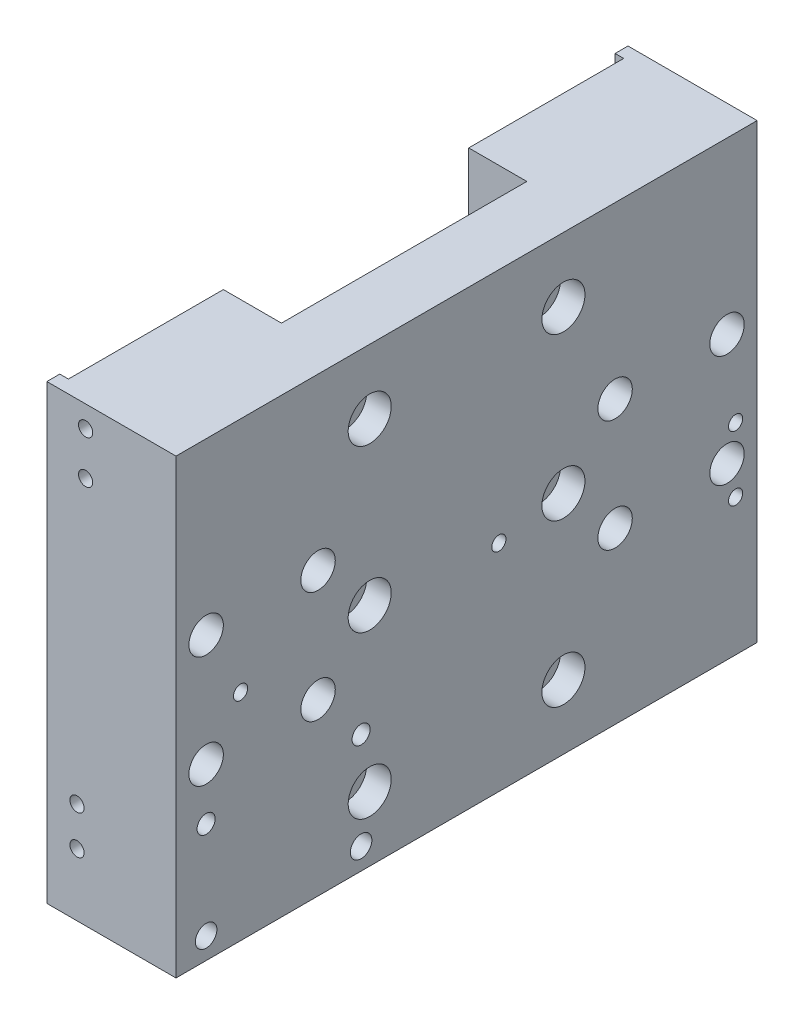
SolidWorks part; units mm, degrees
material "AL6061"
ref_plane "Front Plane" through (0, 0, 0) normal (0, 0, 1) x (1, 0, 0)
ref_plane "Top Plane" through (0, 0, 0) normal (0, 1, 0) x (1, 0, 0)
ref_plane "Right Plane" through (0, 0, 0) normal (1, 0, 0) x (0, 0, -1)
sketch "Sketch1" plane through (0, 0, 0) normal (1, 0, 0) x (0, 0, -1)
  line L1 (-67.5, -52.5) -> (67.5, -52.5)
  line L2 (-67.5, -52.5) -> (-67.5, 52.5)
  line L3 (-67.5, 52.5) -> (67.5, 52.5)
  line L4 (67.5, -52.5) -> (67.5, 52.5)
  line L5 (-67.5, -52.5) -> (67.5, 52.5) construction
  line L6 (-67.5, 52.5) -> (67.5, -52.5) construction
  point P0 (0, 0)
  dimension "D1" = 105
  dimension "D2" = 135
extrude "Boss-Extrude1" add sketch "Sketch1" along normal blind 30
sketch "Sketch2" plane through (0, -52.5, 0) normal (0, -1, 0) x (1, 0, 0)
  line L0 (0, 0) -> (30, 0) construction
  line L2 (0, 67.5) -> (0, -67.5) construction
  line L3 (15.5, -28.5) -> (0, -28.5)
  line L4 (15.5, -28.5) -> (15.5, 28.5)
  line L5 (15.5, 28.5) -> (0, 28.5)
  line L6 (0, -28.5) -> (0, 28.5)
  line L7 (15.5, -28.5) -> (0, 28.5) construction
  line L8 (15.5, 28.5) -> (0, -28.5) construction
  point P5 (7.75, 0)
  dimension "D1" = 57
  dimension "D2" = 15.5
extrude "Cut-Extrude1" cut sketch "Sketch2" against normal through all
sketch "Sketch3" plane through (0, 0, 0) normal (-1, 0, 0) x (0, 0, 1)
  line L0 (0, 52.5) -> (0, -52.5) construction
  line L3 (28.5, 52.5) -> (67.5, 52.5) construction
  line L4 (-64.5, -52.5) -> (64.5, -52.5)
  line L5 (-64.5, -52.5) -> (-64.5, 52.5)
  line L6 (-64.5, 52.5) -> (64.5, 52.5)
  line L7 (64.5, -52.5) -> (64.5, 52.5)
  line L8 (-64.5, -52.5) -> (64.5, 52.5) construction
  line L9 (-64.5, 52.5) -> (64.5, -52.5) construction
  point P6 (0, 0)
  dimension "D1" = 129
extrude "Cut-Extrude2" cut sketch "Sketch3" against normal blind 2
hole_wizard "CBORE for M5 Hexagon socket head cap screws1" positions "Sketch16" profile "Sketch17" counterbore size "M5" standard "GB" end condition through all
sketch "Sketch16" plane through (30, 0, 0) normal (1, 0, 0) x (0, 0, -1)
  line L0 (0, 52.5) -> (0, -52.5) construction
  line L1 (67.5, 52.5) -> (-67.5, 52.5) construction
  line L2 (-67.5, -52.5) -> (67.5, -52.5) construction
  line L3 (67.5, 0) -> (-67.5, 0) construction
  line L4 (67.5, -52.5) -> (67.5, 52.5) construction
  line L5 (-67.5, 52.5) -> (-67.5, -52.5) construction
  point P9 (22.5, 37.5)
  point P11 (-22.5, 37.5)
  point P23 (-22.5, 0)
  point P25 (22.5, 0)
  point P30 (-22.5, -37.5)
  point P31 (22.5, -37.5)
  dimension "D1" = 45
  dimension "D2" = 37.5
sketch "Sketch17" plane through (30, -37.5, -22.5) normal (0, 1, 0) x (0, 0, -1)
  line L0 (0, 0) -> (0, 30)
  line L1 (0, 30) -> (2.75, 30)
  line L3 (2.75, 30) -> (2.75, 5.7)
  line L4 (2.75, 5.7) -> (5, 5.7)
  line L5 (5, 5.7) -> (5, 0)
  line L7 (5, 0) -> (0, 0)
  line L11 (0, -6.35) -> (0, 107.95) construction
  dimension "通孔孔直径" = 5.5
  dimension "通孔孔深度" = 30
  dimension "柱形沉头孔直径" = 10
  dimension "柱形沉头孔深度" = 5.7
hole_wizard "CBORE for M4 Hexagon socket head cap screws1" positions "Sketch22" profile "Sketch23" counterbore size "M4" standard "GB" end condition through all
sketch "Sketch22" plane through (30, 0, 0) normal (1, 0, 0) x (0, 0, -1)
  line L0 (67.5, 0) -> (-67.5, 0) construction
  line L1 (67.5, -52.5) -> (67.5, 52.5) construction
  line L2 (-67.5, 52.5) -> (-67.5, -52.5) construction
  line L4 (0, 52.5) -> (0, -52.5) construction
  line L5 (67.5, 52.5) -> (-67.5, 52.5) construction
  line L6 (-67.5, -52.5) -> (67.5, -52.5) construction
  point P17 (60.5, 13)
  point P19 (60.5, -13)
  point P21 (34.5, -13)
  point P23 (34.5, 13)
  dimension "D1" = 7
  dimension "D2" = 26
  dimension "D3" = 26
sketch "Sketch23" plane through (30, 13, -34.5) normal (0, 1, 0) x (0, 0, -1)
  line L0 (0, 0) -> (0, 30)
  line L1 (0, 30) -> (2.25, 30)
  line L3 (2.25, 30) -> (2.25, 23)
  line L4 (2.25, 23) -> (4, 23)
  line L5 (4, 23) -> (4, 0)
  line L7 (4, 0) -> (0, 0)
  line L11 (0, -6.35) -> (0, 107.95) construction
  dimension "通孔孔直径" = 4.5
  dimension "通孔孔深度" = 30
  dimension "柱形沉头孔直径" = 8
  dimension "柱形沉头孔深度" = 23
mirror "Mirror1" about plane through (0, 0, 0) normal (0, 0, 1) of "CBORE for M4 Hexagon socket head cap screws1"
hole_wizard "M4 Tapped Hole1" positions "Sketch26" profile "Sketch27" tap size "M4" standard "GB"
sketch "Sketch26" plane through (30, 0, 0) normal (1, 0, 0) x (0, 0, -1)
  line L0 (-67.5, -52.5) -> (67.5, -52.5) construction
  line L1 (67.5, -52.5) -> (67.5, 52.5) construction
  point P0 (62.5, -5.75)
  point P3 (62.5, -20.75)
  dimension "D1" = 15
  dimension "D2" = 31.75
  dimension "D3" = 5
sketch "Sketch27" plane through (30, -5.75, -62.5) normal (0, 1, 0) x (0, 0, -1)
  line L0 (0, 0) -> (0, 11.0914)
  line L1 (0, 11.0914) -> (1.65, 10.1)
  line L2 (1.65, 10.1) -> (1.65, 0)
  line L5 (1.65, 0) -> (0, 0)
  line L10 (0, 11.0914) -> (-1.65, 10.1) construction
  line L11 (0, -6.35) -> (0, 107.95) construction
  dimension "螺纹孔钻头直径" = 3.3
  dimension "螺纹孔钻头深度" = 10.1
  dimension "导头角度" = 118
cosmetic thread "Cosmetic Thread7" parameters "D1"=8, "D2"=4
cosmetic thread "Cosmetic Thread17" parameters "D1"=8, "D2"=4
hole_wizard "M6 Tapped Hole1" positions "Sketch30" profile "Sketch29" tap size "M6" standard "GB"
sketch "Sketch30" plane through (0, 0, -67.5) normal (0, 0, -1) x (-1, 0, 0)
  line L0 (0, -52.5) -> (0, 52.5) construction
  line L1 (-30, 52.5) -> (0, 52.5) construction
  point P0 (-12, 42.5)
  point P3 (-12, 22.5)
  dimension "D1" = 12
  dimension "D2" = 10
  dimension "D3" = 20
sketch "Sketch29" plane through (12, 42.5, -67.5) normal (1, 0, 0) x (0, 1, 0)
  line L0 (0, 0) -> (0, 16.5022)
  line L1 (0, 16.5022) -> (2.5, 15)
  line L2 (2.5, 15) -> (2.5, 0)
  line L5 (2.5, 0) -> (0, 0)
  line L10 (0, 16.5022) -> (-2.5, 15) construction
  line L11 (0, -6.35) -> (0, 107.95) construction
  dimension "螺纹孔钻头直径" = 5
  dimension "螺纹孔钻头深度" = 15
  dimension "导头角度" = 118
cosmetic thread "Cosmetic Thread18" parameters "D1"=12, "D2"=6
cosmetic thread "Cosmetic Thread19" parameters "D1"=12, "D2"=6
hole_wizard "M4 Tapped Hole2" positions "Sketch31" profile "Sketch32" tap size "M4" standard "GB"
sketch "Sketch31" plane through (0, 0, 67.5) normal (0, 0, 1) x (1, 0, 0)
  line L0 (11, 47.5) -> (7, 47.5) construction
  line L2 (11, 37.5) -> (7, 37.5) construction
  point P12 (9, 47.5)
  point P14 (9, 37.5)
sketch "Sketch32" plane through (9, 37.5, 67.5) normal (1, 0, 0) x (0, -1, 0)
  line L0 (0, 0) -> (0, 11.0914)
  line L1 (0, 11.0914) -> (1.65, 10.1)
  line L2 (1.65, 10.1) -> (1.65, 0)
  line L5 (1.65, 0) -> (0, 0)
  line L10 (0, 11.0914) -> (-1.65, 10.1) construction
  line L11 (0, -6.35) -> (0, 107.95) construction
  dimension "螺纹孔钻头直径" = 3.3
  dimension "螺纹孔钻头深度" = 10.1
  dimension "导头角度" = 118
cosmetic thread "Cosmetic Thread20" parameters "D1"=8, "D2"=4.3
cosmetic thread "Cosmetic Thread21" parameters "D1"=8, "D2"=4.3
hole_wizard "M4 Tapped Hole3" positions "Sketch33" profile "Sketch34" tap size "M4" standard "GB"
sketch "Sketch33" plane through (0, 0, 67.5) normal (0, 0, 1) x (1, 0, 0)
  point P0 (7, -29)
  point P3 (7, -38)
sketch "Sketch34" plane through (7, -29, 67.5) normal (1, 0, 0) x (0, -1, 0)
  line L0 (0, 0) -> (0, 11.0914)
  line L1 (0, 11.0914) -> (1.65, 10.1)
  line L2 (1.65, 10.1) -> (1.65, 0)
  line L5 (1.65, 0) -> (0, 0)
  line L10 (0, 11.0914) -> (-1.65, 10.1) construction
  line L11 (0, -6.35) -> (0, 107.95) construction
  dimension "螺纹孔钻头直径" = 3.3
  dimension "螺纹孔钻头深度" = 10.1
  dimension "导头角度" = 118
cosmetic thread "Cosmetic Thread13" parameters "D1"=8, "D2"=4
cosmetic thread "Cosmetic Thread14" parameters "D1"=8, "D2"=4
hole_wizard "M5 Tapped Hole1" positions "Sketch35" profile "Sketch36" tap size "M5" standard "GB"
sketch "Sketch35" plane through (30, 0, 0) normal (1, 0, 0) x (0, 0, -1)
  point P0 (-24.5, -25)
  point P3 (-60.5, -25)
sketch "Sketch36" plane through (30, -25, 24.5) normal (0, 1, 0) x (0, 0, -1)
  line L0 (0, 0) -> (0, 13.6618)
  line L1 (0, 13.6618) -> (2.1, 12.4)
  line L2 (2.1, 12.4) -> (2.1, 0)
  line L5 (2.1, 0) -> (0, 0)
  line L10 (0, 13.6618) -> (-2.1, 12.4) construction
  line L11 (0, -6.35) -> (0, 107.95) construction
  dimension "螺纹孔钻头直径" = 4.2
  dimension "螺纹孔钻头深度" = 12.4
  dimension "导头角度" = 118
hole_wizard "Ø5.0mm Dowel Hole1" positions "Sketch37" profile "Sketch38" hole size "Ø5.0" standard "GB"
sketch "Sketch37" plane through (30, 0, 0) normal (1, 0, 0) x (0, 0, -1)
  point P0 (-24.5, -47.5)
  point P3 (-60.5, -47.5)
sketch "Sketch38" plane through (30, -47.5, 24.5) normal (0, 1, 0) x (0, 0, -1)
  line L0 (0, 0) -> (0, 7.5022)
  line L1 (0, 7.5022) -> (2.5, 6)
  line L2 (2.5, 6) -> (2.5, 0)
  line L5 (2.5, 0) -> (0, 0)
  line L10 (0, 7.5022) -> (-2.5, 6) construction
  line L11 (0, -6.35) -> (0, 107.95) construction
  dimension "孔直径" = 5
  dimension "孔深度" = 6
  dimension "导头角度" = 118
hole_wizard "M4 Tapped Hole4" positions "Sketch39" profile "Sketch40" tap size "M4" standard "GB"
sketch "Sketch39" plane through (30, 0, 0) normal (1, 0, 0) x (0, 0, -1)
  line L0 (67.5, 52.5) -> (-67.5, 52.5) construction
  line L1 (-67.5, 52.5) -> (-67.5, -52.5) construction
  point P0 (7.5, -2.5)
  point P2 (-52.5, -2.5)
  dimension "D1" = 55
  dimension "D2" = 15
  dimension "D3" = 60
sketch "Sketch40" plane through (30, -2.5, -7.5) normal (0, 1, 0) x (0, 0, -1)
  line L0 (0, 0) -> (0, 11.0914)
  line L1 (0, 11.0914) -> (1.65, 10.1)
  line L2 (1.65, 10.1) -> (1.65, 0)
  line L5 (1.65, 0) -> (0, 0)
  line L10 (0, 11.0914) -> (-1.65, 10.1) construction
  line L11 (0, -6.35) -> (0, 107.95) construction
  dimension "螺纹孔钻头直径" = 3.3
  dimension "螺纹孔钻头深度" = 10.1
  dimension "导头角度" = 118
cosmetic thread "Cosmetic Thread22" parameters "D1"=8, "D2"=4
cosmetic thread "Cosmetic Thread23" parameters "D1"=8, "D2"=4
